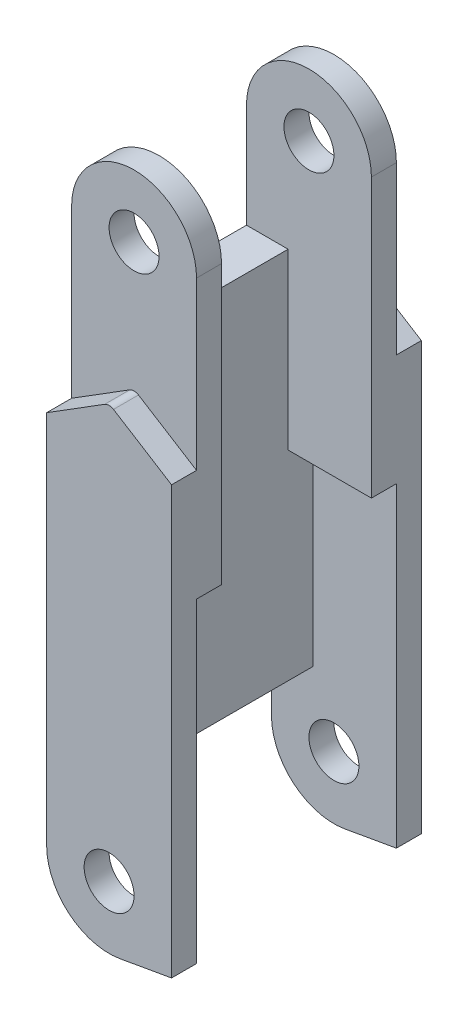
from build123d import *

# Parameters (mm, degrees)
SKETCH1_R           = 3
BOSS_EXTRUDE1_DEPTH = 30
SKETCH2_W           = 24
SKETCH2_H           = 30
SKETCH2_W_2         = 18
SKETCH2_H_2         = 40
CUT_EXTRUDE1_DEPTH  = 42
CUT_EXTRUDE2_DEPTH  = 3
CUT_EXTRUDE3_START  = -30
CUT_EXTRUDE3_DEPTH  = 3
FILLET1_R           = 1
CUT_EXTRUDE4_DEPTH  = 10


with BuildPart() as part:
    # Sketch1 → Boss-Extrude1 (new body)
    with BuildSketch(Plane.XY):
        with BuildLine():
            Line((-7.5, 65), (-7.5, 0))
            ThreePointArc((-7.5, 0), (-4.820907073, -5.745333323), (1.302361333, -7.386058148))
            Line((1.302361333, -7.386058148), (7.5, -6.293247234))
            Line((7.5, -6.293247234), (7.5, 65))
            ThreePointArc((7.5, 65), (0, 72.5), (-7.5, 65))
        make_face()
        Circle(SKETCH1_R, mode=Mode.SUBTRACT)
        with Locations((0, 65)):
            Circle(SKETCH1_R, mode=Mode.SUBTRACT)
    extrude(amount=BOSS_EXTRUDE1_DEPTH)

    # Sketch2 → Cut-Extrude1 (cut)
    with BuildSketch(Plane(origin=(7.5, 0, 0), x_dir=(0, 0, -1), z_dir=(1, 0, 0))):
        with Locations((-15, -7.386058148)):
            Rectangle(SKETCH2_W, SKETCH2_H)
        with Locations((-15, 72.5)):
            Rectangle(SKETCH2_W_2, SKETCH2_H_2)
    extrude(amount=-CUT_EXTRUDE1_DEPTH, mode=Mode.SUBTRACT)

    # Sketch3<2> → Cut-Extrude2 (cut)
    with BuildSketch(Plane.XY.offset(30)):
        Polygon((-7.5, 45), (0, 49.686520139), (7.5, 45), (7.5, 48.622120254), (18.624271708, 48.622120254), (18.624271708, 113.745401459), (-18.624271708, 113.745401459), (-18.624271708, 48.622120254), (-7.5, 48.622120254), align=None)
    extrude(amount=-CUT_EXTRUDE2_DEPTH, mode=Mode.SUBTRACT)

    # 草图3<2> → Cut-Extrude3 (cut)
    with BuildSketch(Plane.XY.offset(30).offset(CUT_EXTRUDE3_START)):
        Polygon((-7.5, 45), (0, 49.686520139), (7.5, 45), (7.5, 48.622120254), (18.624271708, 48.622120254), (18.624271708, 113.745401459), (-18.624271708, 113.745401459), (-18.624271708, 48.622120254), (-7.5, 48.622120254), align=None)
    extrude(amount=CUT_EXTRUDE3_DEPTH, mode=Mode.SUBTRACT)

    # Fillet1
    fillet1_edges = [part.edges().sort_by_distance(p)[0] for p in [
        (0, 49.686520139, 1.5),
        (0, 49.686520139, 28.5),
    ]]
    fillet(fillet1_edges, radius=FILLET1_R)

    # Sketch4 → Cut-Extrude4 (cut)
    with BuildSketch(Plane(origin=(7.5, 0, 0), x_dir=(0, 0, -1), z_dir=(1, 0, 0))):
        Polygon((-3, -16.386058148), (-27, -16.386058148), (-27, 31.613941852), (-24, 31.613941852), (-24, 73.386058148), (-6, 73.386058148), (-6, 31.613941852), (-3, 31.613941852), align=None)
    extrude(amount=-CUT_EXTRUDE4_DEPTH, mode=Mode.SUBTRACT)


solid = part.part
